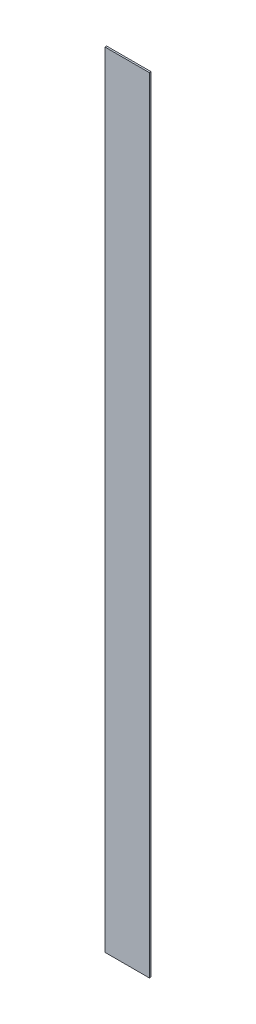
SolidWorks part; units mm, degrees
material "PMMA(有机玻璃)"
ref_plane "前视" through (0, 0, 0) normal (0, 0, 1) x (1, 0, 0)
ref_plane "上视" through (0, 0, 0) normal (0, 1, 0) x (1, 0, 0)
ref_plane "右视" through (0, 0, 0) normal (1, 0, 0) x (0, 0, -1)
sketch "草图1" plane through (0, 0, 0) normal (0, 0, 1) x (1, 0, 0)
  line L1 (-65.5, 1155) -> (65.5, 1155)
  line L2 (-65.5, 1155) -> (-65.5, -1155)
  line L3 (-65.5, -1155) -> (65.5, -1155)
  line L4 (65.5, 1155) -> (65.5, -1155)
  line L5 (-65.5, 1155) -> (65.5, -1155) construction
  line L6 (-65.5, -1155) -> (65.5, 1155) construction
  point P0 (0, 0)
  dimension "D1" = 2310
  dimension "D2" = 131
extrude "凸台-拉伸1" add sketch "草图1" along normal blind 5
hole_wizard "M5 间隙孔1" positions "草图3" profile "草图2" hole size "M5" standard "GB"
sketch "草图3" plane through (0, 0, 5) normal (0, 0, 1) x (1, 0, 0)
  line L0 (-427.5, 273) -> (-427.5, -273) construction
  line L1 (-427.5, -273) -> (427.5, -273) construction
  line L2 (0, 273) -> (0, -273) construction
  line L3 (427.5, 273) -> (-427.5, 273) construction
  line L5 (-427.5, 0) -> (427.5, 0) construction
  line L6 (427.5, -273) -> (427.5, 273) construction
  point P0 (-375, -261)
  point P46 (415.5, 250)
  point P48 (-415.5, 250)
  point P58 (-125, -261)
  point P59 (125, -261)
  point P61 (-125, 261)
  point P62 (125, 261)
  point P64 (-375, 261)
  point P88 (375, -261)
  point P89 (375, 261)
  point P108 (415.5, 0)
  point P109 (-415.5, 0)
  point P110 (415.5, -250)
  point P111 (-415.5, -250)
  dimension "D1" = 12
  dimension "D2" = 12
  dimension "D5" = 3
  dimension "D3" = 12
  dimension "D6" = 4
  dimension "D4" = 2
sketch "草图2" plane through (-375, -261, 5) normal (1, 0, 0) x (0, -1, 0)
  line L0 (0, 0) -> (0, 5)
  line L1 (0, 5) -> (2.75, 5)
  line L2 (2.75, 5) -> (2.75, 0)
  line L5 (2.75, 0) -> (0, 0)
  line L11 (0, -6.35) -> (0, 107.95) construction
  dimension "通孔孔直径" = 5.5
  dimension "通孔孔深度" = 5
